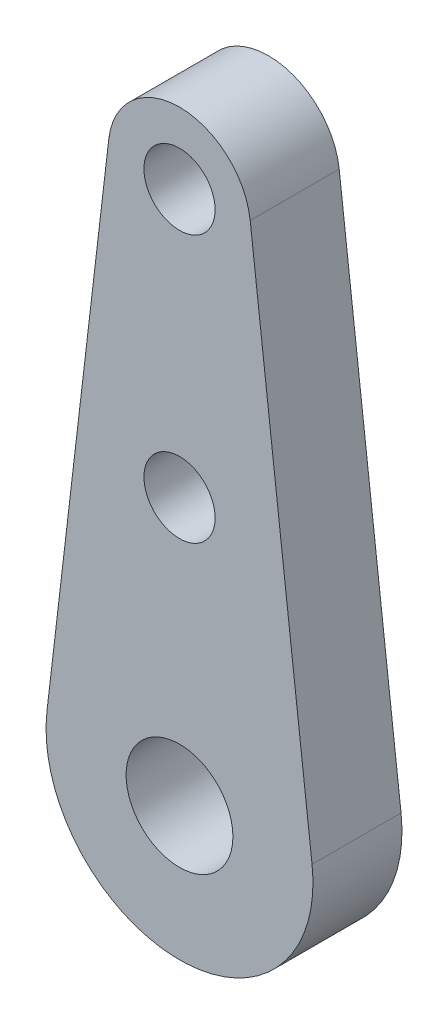
SolidWorks part; units mm, degrees
ref_plane "Front Plane" through (0, 0, 0) normal (0, 0, 1) x (1, 0, 0)
ref_plane "Top Plane" through (0, 0, 0) normal (0, 1, 0) x (1, 0, 0)
ref_plane "Right Plane" through (0, 0, 0) normal (1, 0, 0) x (0, 0, -1)
other "Configuration Table"
sketch "Sketch1" plane through (0, 0, 0) normal (0, 0, 1) x (1, 0, 0)
  line L0 (0, 0) -> (0, 30) construction
  line L1 (-3.9727, 30.4667) -> (-7.4488, 0.875)
  line L2 (3.9727, 30.4667) -> (7.4488, 0.875)
  arc A0 (3.9727, 30.4667) -> (-3.9727, 30.4667) centre (0, 30) ccw
  arc A1 (-7.4488, 0.875) -> (7.4488, 0.875) centre (0, 0) ccw
  circle A2 centre (0, 30) radius 2
  circle A3 centre (0, 0) radius 3
  dimension "D2" = 8
  dimension "D3" = 15
  dimension "D4" = 4
  dimension "D5" = 6
  dimension "D1" = 30
extrude "Boss-Extrude1" add sketch "Sketch1" along normal blind 5
sketch "Sketch2" plane through (0, 0, 5) normal (0, 0, 1) x (1, 0, 0)
  circle A0 centre (0, 15) radius 2
  circle A1 centre (0, 0) radius 3 construction
  dimension "D1" = 4
  dimension "D2" = 15
extrude "Cut-Extrude1" cut sketch "Sketch2" against normal through all
